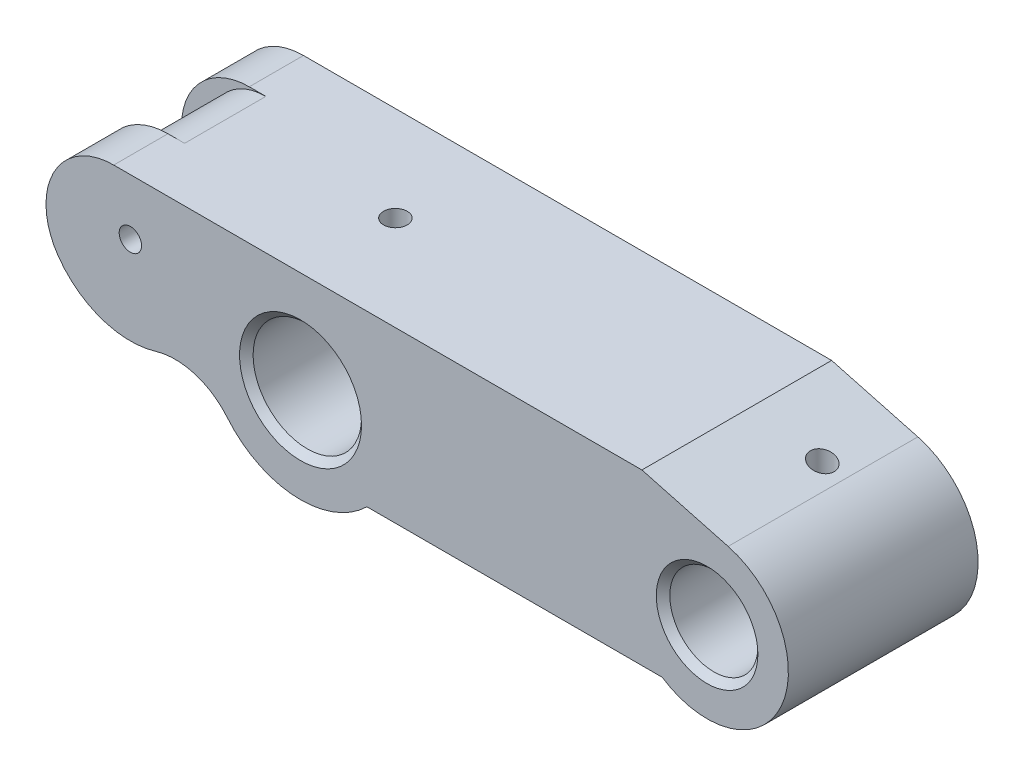
from build123d import *

# Parameters (mm, degrees)
SKETCH1_R               = 8
SKETCH1_R_2             = 6.5
SKETCH1_R_3             = 1.5
BOSS_EXTRUDE1_DEPTH     = 6
SKETCH2_R               = 6.5
SKETCH2_R_2             = 8
BOSS_EXTRUDE2_DEPTH     = 8
CUT_EXTRUDE1_REACH      = 80.873
CUT_EXTRUDE1_END_RADIUS = 8
SKETCH4_R               = 1.75
CUT_EXTRUDE2_REACH      = 80.873
CUT_EXTRUDE2_END_RADIUS = 6.5
SKETCH5_R               = 1.75
CHAMFER1_SIZE           = 1


with BuildPart() as part:
    # Sketch1 → Boss-Extrude1 (new, symmetric)
    with BuildSketch(Plane.XY):
        with BuildLine():
            Line((9.797958971, -10), (53.366750419, -10))
            ThreePointArc((53.366750419, -10), (70.93867824, -4.934097522), (63.105828541, 11.591109915))
            Line((63.105828541, 11.591109915), (50.382575949, 15.000295173))
            Line((50.382575949, 15.000295173), (-25.114071484, 15.000295173))
            ThreePointArc((-25.114071484, 15.000295173), (-33.338477244, 5.852602019), (-23.370562784, -1.355852842))
            ThreePointArc((-23.370562784, -1.355852842), (-17.0207139, -2.075403858), (-12.40317439, -6.493170646))
            ThreePointArc((-12.40317439, -6.493170646), (-2.184319087, -13.828548374), (9.797958971, -10))
        make_face()
        Circle(SKETCH1_R, mode=Mode.SUBTRACT)
        with Locations((60, 0)):
            Circle(SKETCH1_R_2, mode=Mode.SUBTRACT)
        with Locations((-25.114071484, 6.729295173)):
            Circle(SKETCH1_R_3, mode=Mode.SUBTRACT)
    extrude(amount=BOSS_EXTRUDE1_DEPTH, both=True)

    # Sketch2 → Boss-Extrude2 (add)
    with BuildSketch(Plane.XY.offset(6)):
        with BuildLine():
            Line((50.382575949, 15.000295173), (-27.565715626, 15.000295173))
            ThreePointArc((-27.565715626, 15.000295173), (-36.443590747, 9.602830706), (-35.737862766, -0.763038161))
            ThreePointArc((-35.737862766, -0.763038161), (-29.354690281, -5.559608449), (-21.371826468, -5.720427806))
            ThreePointArc((-21.371826468, -5.720427806), (-15.596757504, -5.725786931), (-10.787686266, -8.923330377))
            ThreePointArc((-10.787686266, -8.923330377), (-0.731228007, -13.98089073), (9.797958971, -10))
            Line((9.797958971, -10), (53.366750419, -10))
            ThreePointArc((53.366750419, -10), (70.93867824, -4.934097522), (63.105828541, 11.591109915))
            Line((63.105828541, 11.591109915), (50.382575949, 15.000295173))
        make_face()
        with Locations((60, 0)):
            Circle(SKETCH2_R, mode=Mode.SUBTRACT)
        Circle(SKETCH2_R_2, mode=Mode.SUBTRACT)
    boss_extrude2 = extrude(amount=BOSS_EXTRUDE2_DEPTH)

    # Mirror1: Boss-Extrude2 across plane
    add(boss_extrude2.mirror(Plane.XY))

    # Sketch3 → M4 Tapped Hole1 (revolve, cut)
    with BuildSketch(Plane(origin=(-25.114071484, 6.729295173, 14), x_dir=(0, -1, 0), z_dir=(1, 0, 0))):
        Polygon((0, 0), (0, 8.991420021), (1.65, 8), (1.65, 0), align=None)
    m4_tapped_hole1 = revolve(axis=Axis((-25.114071484, 6.729295173, 20.35), (0, 0, -1)), mode=Mode.SUBTRACT)

    # Mirror2: M4 Tapped Hole1 across plane
    add(m4_tapped_hole1.mirror(Plane.XY), mode=Mode.SUBTRACT)

    # Cut-Extrude1: up to this cylinder (the profile starts outside it)
    cut_extrude1_end = Plane(origin=(0, 0, 0), z_dir=(0, 0, -1)) * Cylinder(CUT_EXTRUDE1_END_RADIUS, 178.746, mode=Mode.PRIVATE)
    # Sketch4 → Cut-Extrude1 (cut, up to the surface)
    with BuildSketch(Plane(origin=(0, 15.000295173, 0), x_dir=(1, 0, 0), z_dir=(0, 1, 0)), mode=Mode.PRIVATE) as cut_extrude1_sk1:
        with Locations(Location((0, 0, 0), (0, 0, 180))):
            Circle(SKETCH4_R)
    cut_extrude1_tool1 = extrude(cut_extrude1_sk1.sketch, amount=-CUT_EXTRUDE1_REACH, mode=Mode.PRIVATE) - cut_extrude1_end
    add(cut_extrude1_tool1.solids().sort_by_distance((0, 15.000295, 0))[0], mode=Mode.SUBTRACT)

    # Cut-Extrude2: up to this cylinder (the profile starts outside it)
    cut_extrude2_end = Plane(origin=(60, 0, -3), z_dir=(0, 0, -1)) * Cylinder(CUT_EXTRUDE2_END_RADIUS, 175.746, mode=Mode.PRIVATE)
    # Sketch5 → Cut-Extrude2 (cut, up to the surface)
    with BuildSketch(Plane(origin=(0, 15.000295173, 0), x_dir=(1, 0, 0), z_dir=(0, 1, 0)), mode=Mode.PRIVATE) as cut_extrude2_sk1:
        with Locations(Location((60, 3, 0), (0, 0, 180))):
            Circle(SKETCH5_R)
    cut_extrude2_tool1 = extrude(cut_extrude2_sk1.sketch, amount=-CUT_EXTRUDE2_REACH, mode=Mode.PRIVATE) - cut_extrude2_end
    add(cut_extrude2_tool1.solids().sort_by_distance((60, 15.000295, -3))[0], mode=Mode.SUBTRACT)

    # Chamfer1
    chamfer1_edges = [part.edges().sort_by_distance(p)[0] for p in [
        (53.5, 0, 14),
        (-8, 0, 14),
        (-8, 0, -14),
        (53.5, 0, -14),
    ]]
    chamfer(chamfer1_edges, length=CHAMFER1_SIZE)


solid = part.part
